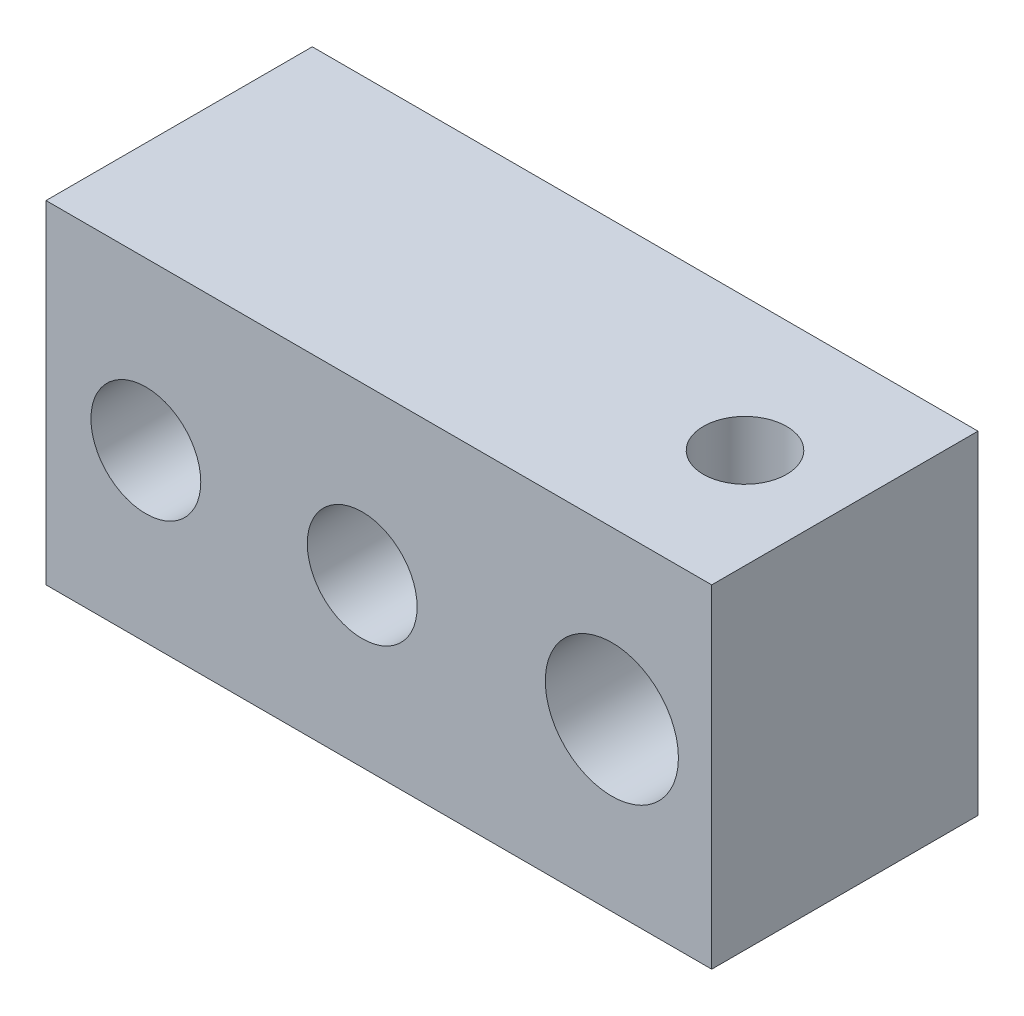
from build123d import *

# Parameters (mm, degrees)
SKETCH_1_W                  = 20
SKETCH_1_H                  = 10
SKETCH_1_R                  = 2
EXTRUDE_1_DEPTH             = 8
SKETCH_2_W                  = 9.758246521
SKETCH_2_H                  = 16.171909484
CUT_EXTRUDE_1_DEPTH         = 22
MOVE_FACE_1_BY              = 7
HOLE_WIZARD_3_3_3_3_1_D     = 3.3
HOLE_WIZARD_3_3_3_3_1_DEPTH = 11.5
HOLE_WIZARD_3_3_3_3_1_TIP   = 0.991420021
HOLE_WIZARD_M3_1_D          = 2.5


with BuildPart() as part:
    # 草图1 → 凸台-拉伸1 (new body)
    with BuildSketch(Plane.XY):
        Rectangle(SKETCH_1_W, SKETCH_1_H)
        Circle(SKETCH_1_R, mode=Mode.SUBTRACT)
    extrude(amount=EXTRUDE_1_DEPTH)

    # 草图2 → 切除-拉伸1 (cut)
    with BuildSketch(Plane(origin=(0, 0, 0), x_dir=(-1, 0, 0), z_dir=(0, 0, -1))):
        with Locations((-7.879123261, 2.238600796)):
            Rectangle(SKETCH_2_W, SKETCH_2_H)
    extrude(amount=-CUT_EXTRUDE_1_DEPTH, mode=Mode.SUBTRACT)

    # Move Face 1: a face moved outward by 7.0
    extrude(part.faces().sort_by_distance((-10, 0, 4))[0], amount=MOVE_FACE_1_BY, dir=(-1, 0, 0))

    # Ø3.3 (3.3) 直径孔1
    with Locations(Plane(origin=(0, 0, 0), x_dir=(-1, 0, 0), z_dir=(0, 0, -1))):
        with Locations((7.5, 0), (14, 0)):
            Hole(HOLE_WIZARD_3_3_3_3_1_D / 2, depth=HOLE_WIZARD_3_3_3_3_1_DEPTH)
            with Locations((0, 0, -(HOLE_WIZARD_3_3_3_3_1_DEPTH + HOLE_WIZARD_3_3_3_3_1_TIP / 2))):  # 118° drill point
                Cone(0, HOLE_WIZARD_3_3_3_3_1_D / 2, HOLE_WIZARD_3_3_3_3_1_TIP, mode=Mode.SUBTRACT)

    # M3 螺纹孔1 (through all)
    with Locations(Plane(origin=(0, 5, 0), x_dir=(1, 0, 0), z_dir=(0, 1, 0))):
        with Locations((0, -4)):
            Hole(HOLE_WIZARD_M3_1_D / 2)


solid = part.part
